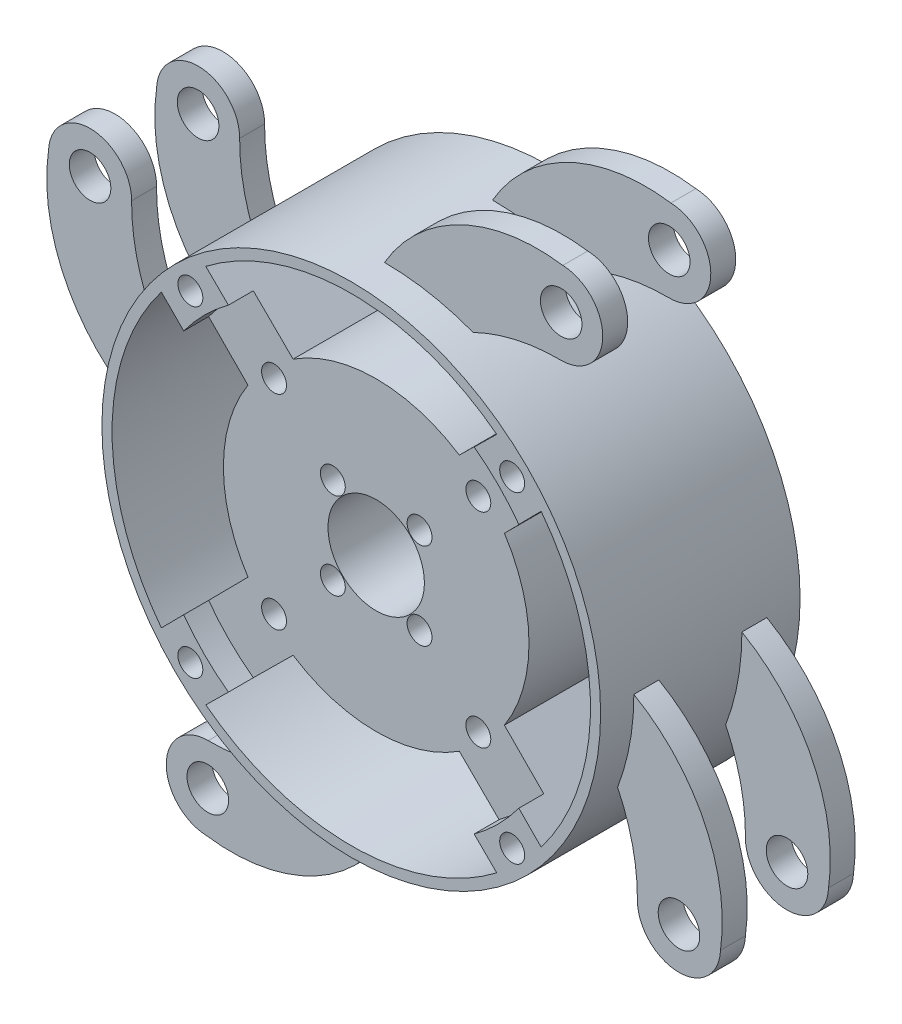
SolidWorks part; units mm, degrees
ref_plane "Front Plane" through (0, 0, 0) normal (0, 0, 1) x (1, 0, 0)
ref_plane "Top Plane" through (0, 0, 0) normal (0, 1, 0) x (1, 0, 0)
ref_plane "Right Plane" through (0, 0, 0) normal (1, 0, 0) x (0, 0, -1)
other "Configuration Table"
sketch "Sketch1" plane through (0, 0, 0) normal (0, 0, 1) x (1, 0, 0)
  circle A0 centre (0, 0) radius 30
  circle A1 centre (0, 0) radius 5.8
  dimension "D1" = 60
  dimension "D2" = 11.6
extrude "Boss-Extrude1" add sketch "Sketch1" along normal mid plane 24
sketch "Sketch2" plane through (0, 0, 12) normal (0, 0, 1) x (1, 0, 0)
  line L0 (0, 0) -> (0, 30) construction
  line L1 (-17.5, 22.8462) -> (-10, 15.4268)
  line L2 (10, 15.4268) -> (17.5, 22.8462)
  line L3 (15.4268, -10) -> (22.8462, -17.5)
  line L4 (22.8462, 17.5) -> (15.4268, 10)
  line L5 (-10, -15.4268) -> (-17.5, -22.8462)
  line L6 (17.5, -22.8462) -> (10, -15.4268)
  line L7 (-15.4268, 10) -> (-22.8462, 17.5)
  line L8 (-22.8462, -17.5) -> (-15.4268, -10)
  circle A0 centre (0, 0) radius 30 construction
  arc A1 (-17.5, 22.8462) -> (17.5, 22.8462) centre (0, 0) cw
  arc A2 (-10, 15.4268) -> (10, 15.4268) centre (0, 0) cw
  arc A3 (22.8462, 17.5) -> (22.8462, -17.5) centre (0, 0) cw
  arc A4 (15.4268, 10) -> (15.4268, -10) centre (0, 0) cw
  arc A5 (17.5, -22.8462) -> (-17.5, -22.8462) centre (0, 0) cw
  arc A6 (10, -15.4268) -> (-10, -15.4268) centre (0, 0) cw
  arc A7 (-22.8462, -17.5) -> (-22.8462, 17.5) centre (0, 0) cw
  arc A8 (-15.4268, -10) -> (-15.4268, 10) centre (0, 0) cw
  point P26 (0, 0)
  dimension "D1" = 20
  dimension "D2" = 35
  dimension "D3" = 17.5
  dimension "D5" = 10
  dimension "D6" = 10
  dimension "D4" = 4
extrude "Cut-Extrude1" cut sketch "Sketch2" against normal through all
sketch "Sketch3" plane through (0, 0, 12) normal (0, 0, 1) x (1, 0, 0)
  line L0 (0, 0) -> (-21.2132, 21.2132) construction
  line L1 (0, 0) -> (0, 30) construction
  circle A0 centre (0, 0) radius 30 construction
  circle A1 centre (-19.3588, 19.3588) radius 1.5
  circle A2 centre (-12.2877, 12.2877) radius 1.5
  circle A3 centre (-5.2167, 5.2167) radius 1.5
  circle A22 centre (19.3588, 19.3588) radius 1.5
  circle A23 centre (12.2877, 12.2877) radius 1.5
  circle A24 centre (5.2167, 5.2167) radius 1.5
  circle A25 centre (19.3588, -19.3588) radius 1.5
  circle A26 centre (12.2877, -12.2877) radius 1.5
  circle A27 centre (5.2167, -5.2167) radius 1.5
  circle A28 centre (-19.3588, -19.3588) radius 1.5
  circle A29 centre (-12.2877, -12.2877) radius 1.5
  circle A30 centre (-5.2167, -5.2167) radius 1.5
  point P33 (2.769, -2.769)
  point P34 (2.7829, -2.7829)
  point P35 (0, 0)
  dimension "D2" = 3
  dimension "D1" = 45
  dimension "D3" = 3
  dimension "D4" = 4
extrude "Cut-Extrude2" cut sketch "Sketch3" against normal through all
sketch "Sketch4" plane through (0, 0, 12) normal (0, 0, 1) x (1, 0, 0)
  circle A0 centre (0, 0) radius 25
  dimension "D1" = 50
extrude "Cut-Extrude3" cut sketch "Sketch4" against normal blind 3
mirror "Mirror1" about plane through (0, 0, 0) normal (0, 0, 1) of "Cut-Extrude3"
sketch "Sketch5" plane through (0, 0, 0) normal (0, 0, 1) x (1, 0, 0)
  line L0 (0, 0) -> (0, 30) construction
  circle A0 centre (0, 0) radius 30 construction
  circle A7 centre (21.2579, 35.4269) radius 2.5
  arc A11 (0, 30) -> (21.456, 40.423) centre (18.4282, 19.3604) cw
  arc A12 (21.456, 40.423) -> (21.2198, 30.4271) centre (21.2579, 35.4269) cw
  arc A13 (21.2198, 30.4271) -> (10.6579, 28.043) centre (21.0387, 6.6416) ccw
  arc A14 (0, 30) -> (10.6579, 28.043) centre (0, 0) cw
  dimension "D1" = 5
  dimension "D6" = 5
extrude "Boss-Extrude2" add sketch "Sketch5" along normal mid plane 16
pattern_circular "CirPattern1" count 4 over 360 about axis through (0, 0, 0) along (0, 0, 1) of "Boss-Extrude2"
sketch "Sketch16" plane through (0, 0, 0) normal (0, 0, 1) x (1, 0, 0)
  arc A0 (-10.6579, -28.043) -> (0, -30) centre (0, 0) ccw construction
  arc A1 (-21.2198, -30.4271) -> (-10.6579, -28.043) centre (-21.0387, -6.6416) ccw construction
  arc A2 (-21.2198, -30.4271) -> (-21.456, -40.423) centre (-21.2579, -35.4269) ccw construction
  arc A3 (-21.456, -40.423) -> (0, -30) centre (-18.4282, -19.3604) ccw construction
  arc A4 (28.043, -10.6579) -> (30, 0) centre (0, 0) ccw construction
  arc A5 (30.4271, -21.2198) -> (28.043, -10.6579) centre (6.6416, -21.0387) ccw construction
  arc A6 (30.4271, -21.2198) -> (40.423, -21.456) centre (35.4269, -21.2579) ccw construction
  arc A7 (40.423, -21.456) -> (30, 0) centre (19.3604, -18.4282) ccw construction
  arc A8 (10.6579, 28.043) -> (0, 30) centre (0, 0) ccw construction
  arc A9 (21.2198, 30.4271) -> (10.6579, 28.043) centre (21.0387, 6.6416) ccw construction
  arc A10 (21.2198, 30.4271) -> (21.456, 40.423) centre (21.2579, 35.4269) ccw construction
  arc A11 (21.456, 40.423) -> (0, 30) centre (18.4282, 19.3604) ccw construction
  arc A12 (-28.043, 10.6579) -> (-30, 0) centre (0, 0) ccw construction
  arc A13 (-30.4271, 21.2198) -> (-28.043, 10.6579) centre (-6.6416, 21.0387) ccw construction
  arc A14 (-30.4271, 21.2198) -> (-40.423, 21.456) centre (-35.4269, 21.2579) ccw construction
  arc A15 (-40.423, 21.456) -> (-30, 0) centre (-19.3604, 18.4282) ccw construction
  arc A16 (-10.6579, -28.043) -> (0, -30) centre (0, 0) ccw
  arc A17 (-21.2198, -30.4271) -> (-10.6579, -28.043) centre (-21.0387, -6.6416) ccw
  arc A18 (-21.2198, -30.4271) -> (-21.456, -40.423) centre (-21.2579, -35.4269) ccw
  arc A19 (-21.456, -40.423) -> (0, -30) centre (-18.4282, -19.3604) ccw
  arc A20 (28.043, -10.6579) -> (30, 0) centre (0, 0) ccw
  arc A21 (30.4271, -21.2198) -> (28.043, -10.6579) centre (6.6416, -21.0387) ccw
  arc A22 (30.4271, -21.2198) -> (40.423, -21.456) centre (35.4269, -21.2579) ccw
  arc A23 (40.423, -21.456) -> (30, 0) centre (19.3604, -18.4282) ccw
  arc A24 (10.6579, 28.043) -> (0, 30) centre (0, 0) ccw
  arc A25 (21.2198, 30.4271) -> (10.6579, 28.043) centre (21.0387, 6.6416) ccw
  arc A26 (21.2198, 30.4271) -> (21.456, 40.423) centre (21.2579, 35.4269) ccw
  arc A27 (21.456, 40.423) -> (0, 30) centre (18.4282, 19.3604) ccw
  arc A28 (-28.043, 10.6579) -> (-30, 0) centre (0, 0) ccw
  arc A29 (-30.4271, 21.2198) -> (-28.043, 10.6579) centre (-6.6416, 21.0387) ccw
  arc A30 (-30.4271, 21.2198) -> (-40.423, 21.456) centre (-35.4269, 21.2579) ccw
  arc A31 (-40.423, 21.456) -> (-30, 0) centre (-19.3604, 18.4282) ccw
extrude "Cut-Extrude11" cut sketch "Sketch16" against normal mid plane 5
scale "Scale 1" bodies to scale 116 scale about origin uniform scaling yes scale factor 0.5
sketch "Sketch17" plane through (0, 0, 0) normal (0, 0, 1) x (1, 0, 0)
  arc A0 (-5.3289, -14.0215) -> (0, -15) centre (0, 0) ccw construction
  arc A1 (-10.6099, -15.2135) -> (-5.3289, -14.0215) centre (-10.5194, -3.3208) ccw construction
  arc A2 (-10.6099, -15.2135) -> (-10.728, -20.2115) centre (-10.629, -17.7135) ccw construction
  arc A3 (-10.728, -20.2115) -> (0, -15) centre (-9.2141, -9.6802) ccw construction
  arc A4 (14.0215, -5.3289) -> (15, 0) centre (0, 0) ccw construction
  arc A5 (15.2135, -10.6099) -> (14.0215, -5.3289) centre (3.3208, -10.5194) ccw construction
  arc A6 (15.2135, -10.6099) -> (20.2115, -10.728) centre (17.7135, -10.629) ccw construction
  arc A7 (20.2115, -10.728) -> (15, 0) centre (9.6802, -9.2141) ccw construction
  arc A8 (5.3289, 14.0215) -> (0, 15) centre (0, 0) ccw construction
  arc A9 (10.6099, 15.2135) -> (5.3289, 14.0215) centre (10.5194, 3.3208) ccw construction
  arc A10 (10.6099, 15.2135) -> (10.728, 20.2115) centre (10.629, 17.7135) ccw construction
  arc A11 (10.728, 20.2115) -> (0, 15) centre (9.2141, 9.6802) ccw construction
  arc A12 (-14.0215, 5.3289) -> (-15, 0) centre (0, 0) ccw construction
  arc A13 (-15.2135, 10.6099) -> (-14.0215, 5.3289) centre (-3.3208, 10.5194) ccw construction
  arc A14 (-15.2135, 10.6099) -> (-20.2115, 10.728) centre (-17.7135, 10.629) ccw construction
  arc A15 (-20.2115, 10.728) -> (-15, 0) centre (-9.6802, 9.2141) ccw construction
  arc A16 (-5.3289, -14.0215) -> (0, -15) centre (0, 0) ccw
  arc A17 (-10.6099, -15.2135) -> (-5.3289, -14.0215) centre (-10.5194, -3.3208) ccw
  arc A18 (-10.6099, -15.2135) -> (-10.728, -20.2115) centre (-10.629, -17.7135) ccw
  arc A19 (-10.728, -20.2115) -> (0, -15) centre (-9.2141, -9.6802) ccw
  arc A20 (14.0215, -5.3289) -> (15, 0) centre (0, 0) ccw
  arc A21 (15.2135, -10.6099) -> (14.0215, -5.3289) centre (3.3208, -10.5194) ccw
  arc A22 (15.2135, -10.6099) -> (20.2115, -10.728) centre (17.7135, -10.629) ccw
  arc A23 (20.2115, -10.728) -> (15, 0) centre (9.6802, -9.2141) ccw
  arc A24 (5.3289, 14.0215) -> (0, 15) centre (0, 0) ccw
  arc A25 (10.6099, 15.2135) -> (5.3289, 14.0215) centre (10.5194, 3.3208) ccw
  arc A26 (10.6099, 15.2135) -> (10.728, 20.2115) centre (10.629, 17.7135) ccw
  arc A27 (10.728, 20.2115) -> (0, 15) centre (9.2141, 9.6802) ccw
  arc A28 (-14.0215, 5.3289) -> (-15, 0) centre (0, 0) ccw
  arc A29 (-15.2135, 10.6099) -> (-14.0215, 5.3289) centre (-3.3208, 10.5194) ccw
  arc A30 (-15.2135, 10.6099) -> (-20.2115, 10.728) centre (-17.7135, 10.629) ccw
  arc A31 (-20.2115, 10.728) -> (-15, 0) centre (-9.6802, 9.2141) ccw
extrude "Cut-Extrude12" cut sketch "Sketch17" against normal mid plane 5
